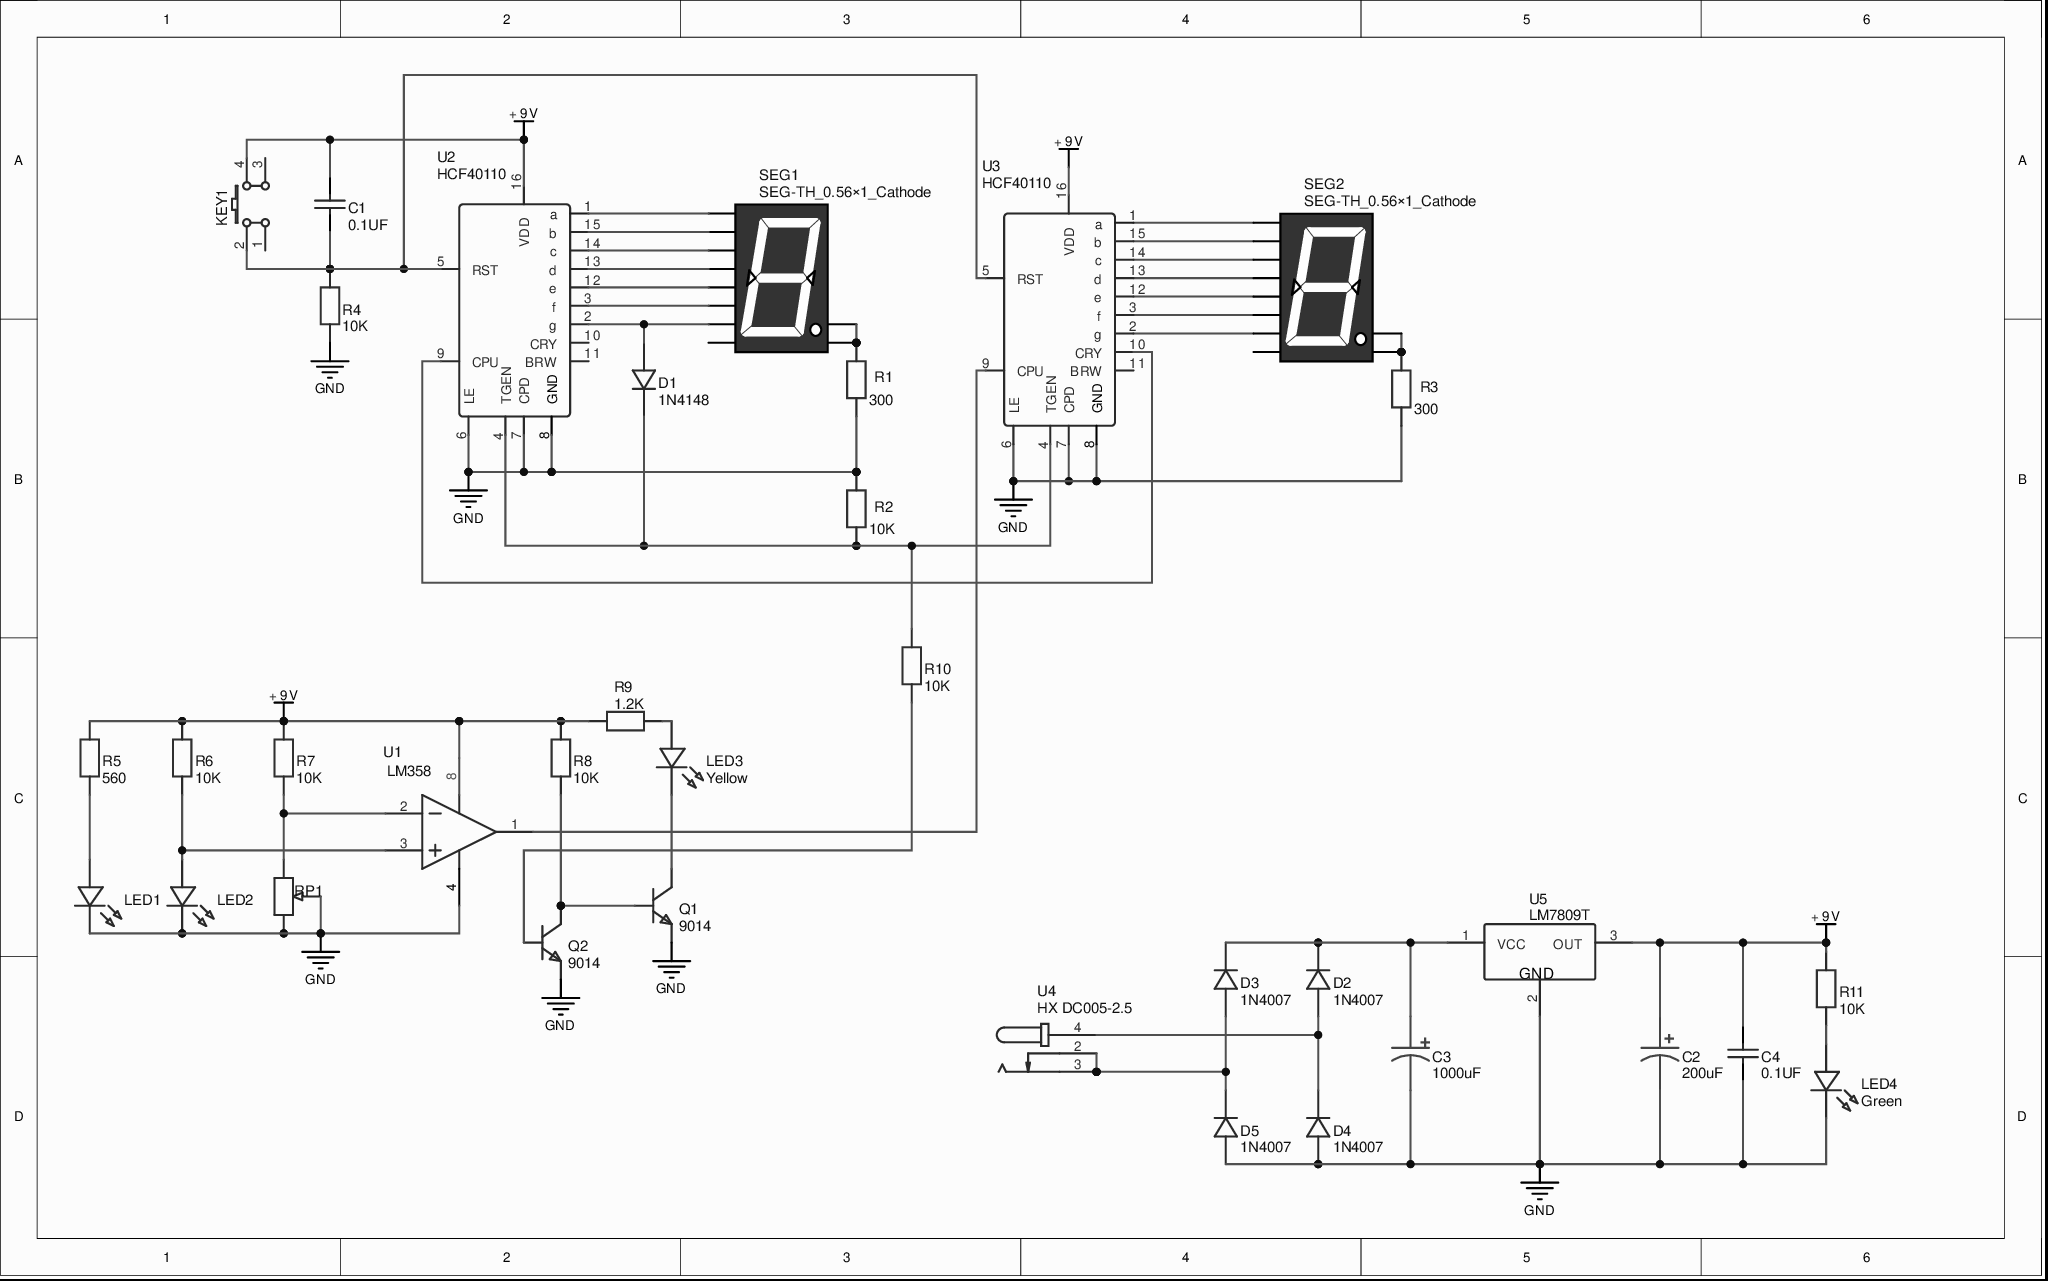
[diagram p0: MISC82671-2.schdoc]
# Altium project MISC82671-5.PrjPcb
1 sheet, 35 parts. Net scope: global (net labels, ports and power ports of the same name join across sheets).
Board file: MISC82671.pcbdoc

## Sheet MISC82671-2.schdoc
size 280 x 175 mm

### Parts
C1  0.1UF  [CAP-TH_L5.0-W4.0-P5.00-D1.0]
C2  200uF  [CAP-TH_BD10.0-P5.00-D1.0-FD]
C3  1000uF  [CAP-TH_BD10.0-P5.00-D1.0-FD]
C4  0.1UF  [CAP-TH_L5.0-W4.0-P5.00-D1.0]
D1  1N4148  [DO-35_BD2.2-L4.0-D0.50_1N4148]
D2  1N4007  [DO-41_BD2.4-L4.7-P8.70-D0.9-FD]
D3  1N4007  [DO-41_BD2.4-L4.7-P8.70-D0.9-FD]
D4  1N4007  [DO-41_BD2.4-L4.7-P8.70-D0.9-FD]
D5  1N4007  [DO-41_BD2.4-L4.7-P8.70-D0.9-FD]
KEY1  K4-6×6_TH  [KEY-TH_4P-L6.0-W6.0-P4.50-LS6.5]  (value not drawn)
LED1  LED-TH-5mm_R  [LED-TH_BD5.0_RED]  (value not drawn)
LED2  LED-TH-5mm_R  [LED-TH_BD5.0_RED]  (value not drawn)
LED3  Yellow  [LED-TH_BD5.0_RED]
LED4  Green  [LED-TH_BD5.0_RED]
Q1  9014  [TO-92-3_L4.9-W3.7-P2.54-L]
Q2  9014  [TO-92-3_L4.9-W3.7-P2.54-L]
R1  300  [R_AXIAL-0.4]
R2  10K  [R_AXIAL-0.4]
R3  300  [R_AXIAL-0.4]
R4  10K  [R_AXIAL-0.4]
R5  560  [R_AXIAL-0.4]
R6  10K  [R_AXIAL-0.4]
R7  10K  [R_AXIAL-0.4]
R8  10K  [R_AXIAL-0.4]
R9  1.2K  [R_AXIAL-0.4]
R10  10K  [R_AXIAL-0.4]
R11  10K  [R_AXIAL-0.4]
RP1  R_3386P_EU  [RES-ADJ-TH_3386P]  (value not drawn)
SEG1  SEG-TH_0.56×1_Cathode  [LED-SEG-TH_10P-L12.6-W19.0-P2.54-S15.24-BL]
SEG2  SEG-TH_0.56×1_Cathode  [LED-SEG-TH_10P-L12.6-W19.0-P2.54-S15.24-BL]
U1  LM358  [DIP-8_L8.8-W6.4-P2.54-LS7.6-BL]
U2  HCF40110  [DIP-16_16P-L20.2-W6.6-P2.54-LS7.6-BL]
U3  HCF40110  [DIP-16_16P-L20.2-W6.6-P2.54-LS7.6-BL]
U4  HX DC005-2.5  [DC-IN-TH_HX-DC005-2.5]
U5  LM7809T  [TO-220-3_L10.0-W4.5-P2.54-L]

### Nets
+9V: C1.2 C2.1 C4.2 KEY1.4 R5.2 R6.2 R7.2 R8.2 R9.2 R11.2 U1.8(V+) U2.16(VDD) U3.16(VDD) U5.3(OUT)
GND: C2.2 C3.2 C4.1 D4.1(A) D5.1(A) LED1.2 LED2.2 LED4.2 Q1.1(E) Q2.1(E) R1.1 R2.2 R3.1 R4.1 RP1.2 RP1.3 U1.4(GND) U2.6(LE) U2.7(CPD) U2.8(GND) U3.6(LE) U3.7(CPD) U3.8(GND) U5.2(GND)
NetC1_1: C1.1 KEY1.2 R4.2 U2.5(RST) U3.5(RST)
NetC3_1: C3.1 D2.2(K) D3.2(K) U5.1(VCC)
NetD1_1: D1.1(A) SEG1.10(G) U2.2(g)
NetD1_2: D1.2(C) R2.1 R10.2 U2.4(TGEN) U3.4(TGEN)
NetD2_1: D2.1(A) D4.2(K) U4.4
NetD3_1: D3.1(A) D5.2(K) U4.2 U4.3
NetLED1_1: LED1.1 R5.1
NetLED2_1: LED2.1 R6.1 U1.3(INA+)
NetLED3_1: LED3.1 R9.1
NetLED3_2: LED3.2 Q1.3(C)
NetLED4_1: LED4.1 R11.1
NetQ1_2: Q1.2(B) Q2.3(C) R8.1
NetQ2_2: Q2.2(B) R10.1
NetR1_2: R1.2 SEG1.3(G1) SEG1.8(G2)
NetR3_2: R3.2 SEG2.3(G1) SEG2.8(G2)
NetR7_1: R7.1 RP1.1 U1.2(INA-)
NetSEG1_1: SEG1.1(E) U2.12(e)
NetSEG1_2: SEG1.2(D) U2.13(d)
NetSEG1_4: SEG1.4(C) U2.14(c)
NetSEG1_6: SEG1.6(B) U2.15(b)
NetSEG1_7: SEG1.7(A) U2.1(a)
NetSEG1_9: SEG1.9(F) U2.3(f)
NetSEG2_1: SEG2.1(E) U3.12(e)
NetSEG2_2: SEG2.2(D) U3.13(d)
NetSEG2_4: SEG2.4(C) U3.14(c)
NetSEG2_6: SEG2.6(B) U3.15(b)
NetSEG2_7: SEG2.7(A) U3.1(a)
NetSEG2_9: SEG2.9(F) U3.3(f)
NetSEG2_10: SEG2.10(G) U3.2(g)
NetU1_1: U1.1(OUTA) U3.9(CPU)
NetU2_9: U2.9(CPU) U3.10(CRY)

Not connected (* = marked no-connect by the designer): KEY1 1* 3*; SEG1 5(DP); SEG2 5(DP); U2 10(CRY) 11(BRW); U3 11(BRW)

### Library data of the parts
C1 C4 = 0.1UF: Manufacturer: null; Manufacturer Part: 瓷片电容47PF 3KV; nameAlias: Value; Supplier: LCSC; Supplier Part: C19375; JLCPCB Part Class: Extended Part; link: https://so.szlcsc.com/global.html?k=C19375&ref=editor; spicePre: C; spiceSymbolName: Ceramic capacitors47PF 3KV
C2 = 200uF: Manufacturer: rubycon(红宝石); Manufacturer Part: 8AX200MEFC6.3X7; Contributor: lcsc; Convert to PCB: Yes; nameAlias: Value; Add into BOM: Yes; Supplier: LCSC; Supplier Part: C5115550; JLCPCB Part Class: Extended Part; link: https://so.szlcsc.com/global.html?k=C5115550&ref=editor; spicePre: C; spiceSymbolName: 8AX200MEFC6.3X7
C3 = 1000uF: Manufacturer: HRK(鸿瑞凯电子); Manufacturer Part: 25V1000uF CD288; Contributor: lcsc; nameAlias: Value; Supplier: LCSC; Supplier Part: C2960265; JLCPCB Part Class: Extended Part; link: https://so.szlcsc.com/global.html?k=C2960265&ref=editor; spicePre: U; spiceSymbolName: 25V-1000UF-CD288
D1 = 1N4148: Manufacturer: null; Contributor: lcsc; Supplier: LCSC; Supplier Part: C9900036548; Manufacturer Part: 1N4148; JLCPCB Part Class: Extended Part; link: https://so.szlcsc.com/global.html?k=C9900036548&ref=editor; spicePre: D; spiceSymbolName: 1N4148_C9900036548
D2-D5 = 1N4007: Manufacturer: VISHAY(威世); Manufacturer Part: 1N4007-E3/54; Supplier: LCSC; Supplier Part: C84643; JLCPCB Part Class: Extended Part; link: https://so.szlcsc.com/global.html?k=C84643&ref=editor; spicePre: D; spiceSymbolName: 1N4007-E3/54
KEY1 = K4-6×6_TH: Manufacturer: 韩国韩荣; Manufacturer Part: K2-1102DP-E4SW-04; Contributor: LCEDA_Lib; Supplier: LCSC; Supplier Part: C136684; spicePre: K; spiceSymbolName: K4-6×6_TH
LED1 LED2 = LED-TH-5mm_R: Manufacturer: EVERLIGHT(台湾亿光); Manufacturer Part: 333-2SURD/S530-A3; Contributor: LCEDA_Lib; Supplier Part: C87271; Supplier: LCSC; spicePre: L; spiceSymbolName: LED-TH-5mm_R
LED3 = 黄: Manufacturer: EVERLIGHT(台湾亿光); Manufacturer Part: 333-2SURD/S530-A3; Contributor: LCEDA_Lib; Supplier Part: C87271; Supplier: LCSC; spicePre: L; spiceSymbolName: LED-TH-5mm_R
LED4 = 绿: Manufacturer: EVERLIGHT(台湾亿光); Manufacturer Part: 333-2SURD/S530-A3; Contributor: LCEDA_Lib; Supplier Part: C87271; Supplier: LCSC; spicePre: L; spiceSymbolName: LED-TH-5mm_R
Q1 Q2 = 9014: Manufacturer: BLUE ROCKET(蓝箭); Contributor: lcsc; Supplier: LCSC; Supplier Part: C3037604; Manufacturer Part: 9014; JLCPCB Part Class: Extended Part; link: https://so.szlcsc.com/global.html?k=C3037604&ref=editor; spicePre: Q; spiceSymbolName: 9014
R1 R3 = 300: nameAlias: Value(Ω); Contributor: LCEDA_Lib; spicePre: R; spiceSymbolName: R_AXIAL-0.4_EU
R2 R4 R6-R8 R10 R11 = 10K: nameAlias: Value(Ω); Contributor: LCEDA_Lib; spicePre: R; spiceSymbolName: R_AXIAL-0.4_EU
R5 = 560: nameAlias: Value(Ω); Contributor: LCEDA_Lib; spicePre: R; spiceSymbolName: R_AXIAL-0.4_EU
R9 = 1.2K: nameAlias: Value(Ω); Contributor: LCEDA_Lib; spicePre: R; spiceSymbolName: R_AXIAL-0.4_EU
RP1 = R_3386P_EU: nameAlias: Resistance (Ohms); Contributor: LCEDA_Lib; Value(Ω): 10K; Supplier: LCSC; spicePre: R; spiceSymbolName: R_3386P_EU
SEG1 SEG2 = SEG-TH_0.56×1_Cathode: Manufacturer: 志浩; Contributor: LCEDA_01; Supplier Part: C8093; spicePre: S; spiceSymbolName: SEG-TH_0.56×1_Cathode
U1 = LM358: Manufacturer Part: TI; subpart_no: 2; Value: LM358MX/NOPB; Contributor: zxk8; Supplier Part: C16416; Supplier: LCSC; Manufacturer: LM358MX/NOPB; JLCPCB Part Class: Extended Part; spicePre: U; spiceSymbolName: LM358MX/NOPB
U2 U3 = HCF40110: Manufacturer: STMicroelectronics; Manufacturer Part: HCF4017BE; Contributor: jtaom; Supplier: LCSC; image: C5166.jpg; Supplier Part: C5166; spicePre: U; spiceSymbolName: HCF40110
U4 = HX DC005-2.5: Manufacturer: hanxia(韩下); Contributor: lcsc; Supplier: LCSC; Supplier Part: C18357599; Manufacturer Part: HX DC005-2.5; JLCPCB Part Class: Extended Part; link: https://so.szlcsc.com/global.html?k=C18357599&ref=editor; spicePre: U; spiceSymbolName: HX DC005-2.5
U5 = LM7809T: Manufacturer: HGSEMI(华冠); Contributor: LCSC; Supplier: LCSC; Supplier Part: C507141; Manufacturer Part: LM7809T; JLCPCB Part Class: Extended Part; link: https://so.szlcsc.com/global.html?k=C507141&ref=editor; spicePre: U; spiceSymbolName: LM7809T